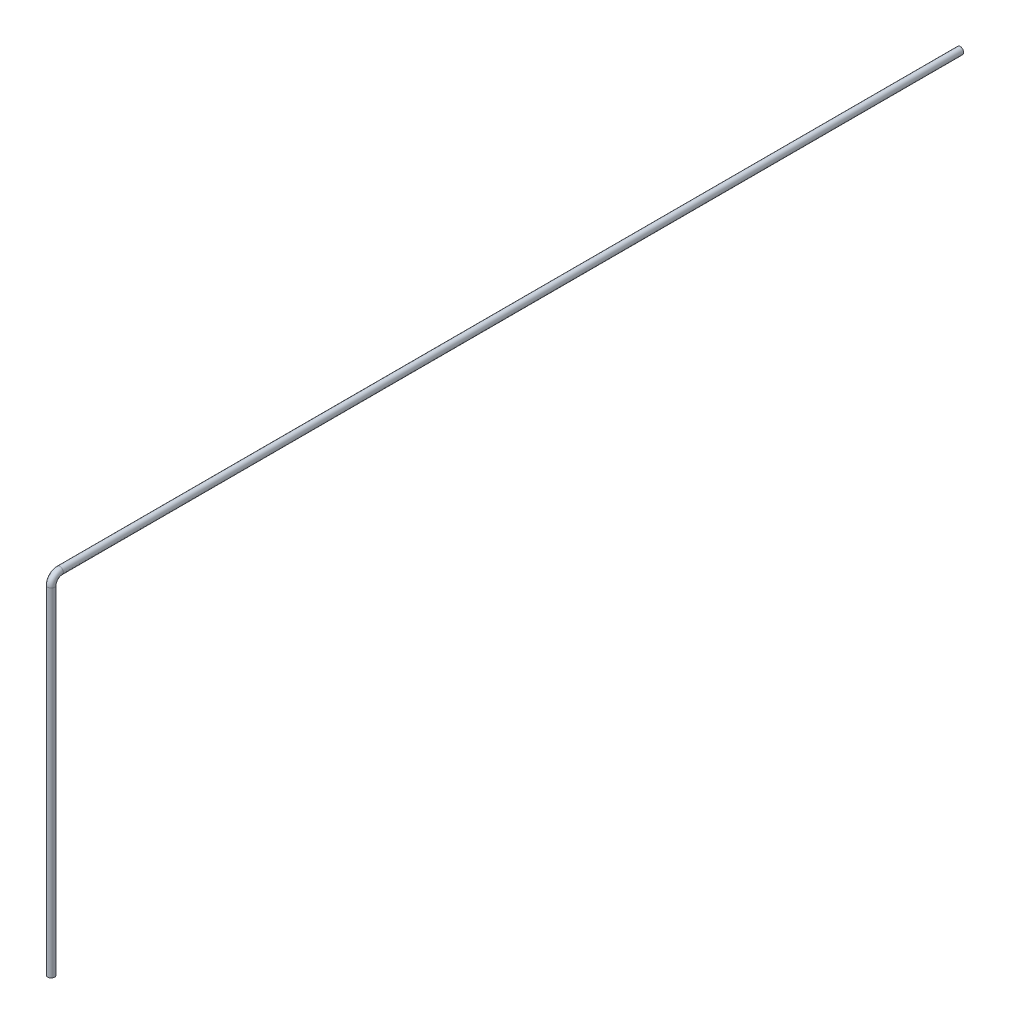
SolidWorks part; units mm, degrees
material "Q235B"
ref_plane "Front Plane" through (0, 0, 0) normal (0, 0, 1) x (1, 0, 0)
ref_plane "Top Plane" through (0, 0, 0) normal (0, 1, 0) x (1, 0, 0)
ref_plane "Right Plane" through (0, 0, 0) normal (1, 0, 0) x (0, 0, -1)
sketch "Sketch1" plane through (0, 0, 0) normal (0, 1, 0) x (1, 0, 0)
  circle A0 centre (0, 0) radius 4
  circle A1 centre (0, 0) radius 3
  dimension "D1" = 8
  dimension "D2" = 6
sketch "Sketch2" plane through (0, 0, 0) normal (1, 0, 0) x (0, 0, -1)
  line L0 (0, 0) -> (0, 390)
  line L1 (10, 400) -> (1050, 400)
  arc A0 (10, 400) -> (0, 390) centre (10, 390) ccw
  point P6 (0, 400)
  dimension "D3" = 10
  dimension "D1" = 400
  dimension "D2" = 1050
sweep "Sweep1" add profiles "Sketch1" path "Sketch2"
